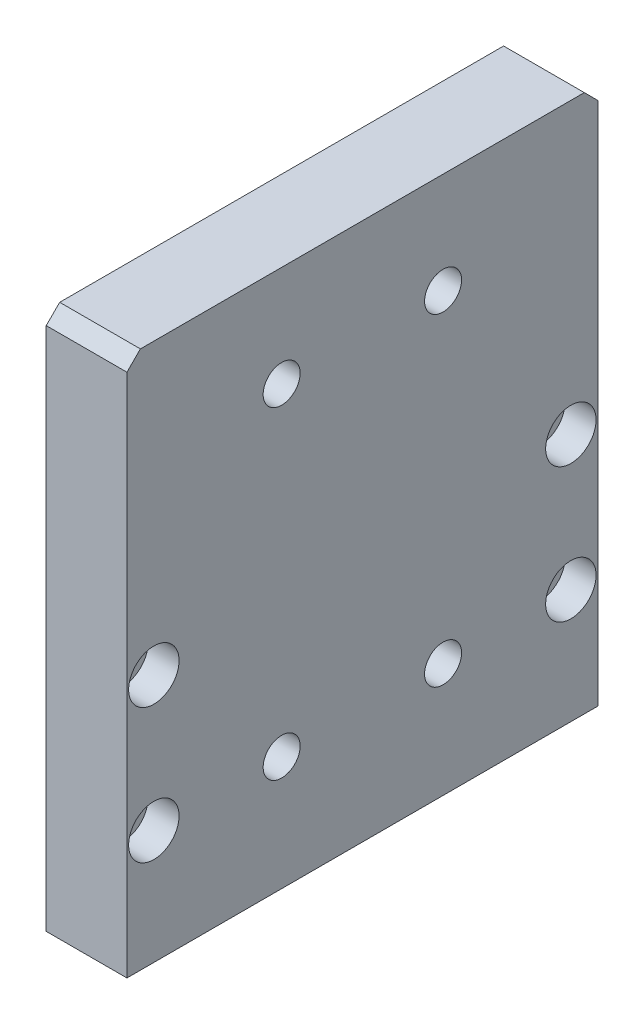
from build123d import *

# Parameters (mm, degrees)
SKETCH_1_W                   = 70
SKETCH_1_H                   = 80
EXTRUDE_1_DEPTH              = 12
HOLE_WIZARD_M5_1_D           = 5.5
HOLE_WIZARD_M5_1_CBORE_D     = 10
HOLE_WIZARD_M5_1_CBORE_DEPTH = 5.7
HOLE_WIZARD_M4_1_D           = 4.5
HOLE_WIZARD_M4_1_CBORE_D     = 7.5
HOLE_WIZARD_M4_1_CBORE_DEPTH = 4.6
HOLE_WIZARD_M4_1_2_D         = 3.3
HOLE_WIZARD_M4_1_2_DEPTH     = 10.1
HOLE_WIZARD_M4_1_2_TIP       = 0.991420021
CHAMFER_1_SIZE               = 2


with BuildPart() as part:
    # 草图1 → 凸台-拉伸1 (new body)
    with BuildSketch(Plane(origin=(0, 0, 0), x_dir=(0, 0, -1), z_dir=(1, 0, 0))):
        Rectangle(SKETCH_1_W, SKETCH_1_H)
    extrude(amount=EXTRUDE_1_DEPTH)

    # M5 六角圆柱头螺钉的柱形沉头孔1 (through all)
    with Locations(Plane.ZY):
        with Locations((-12, 25), (-12, -23), (12, -23), (12, 25)):
            CounterBoreHole(HOLE_WIZARD_M5_1_D / 2, HOLE_WIZARD_M5_1_CBORE_D / 2, HOLE_WIZARD_M5_1_CBORE_DEPTH)

    # Hole Wizard M4 _1 (through all)
    with Locations(Plane(origin=(12, 0, 0), x_dir=(0, 0, -1), z_dir=(1, 0, 0))):
        with Locations((-31, -23), (-31, -3), (31, -3), (31, -23)):
            CounterBoreHole(HOLE_WIZARD_M4_1_D / 2, HOLE_WIZARD_M4_1_CBORE_D / 2, HOLE_WIZARD_M4_1_CBORE_DEPTH)

    # Hole Wizard M4 _1 2
    with Locations(Plane(origin=(0, -40, 0), x_dir=(-1, 0, 0), z_dir=(0, -1, 0))):
        with Locations((-6, 22.5), (-6, -22.5)):
            Hole(HOLE_WIZARD_M4_1_2_D / 2, depth=HOLE_WIZARD_M4_1_2_DEPTH)
            with Locations((0, 0, -(HOLE_WIZARD_M4_1_2_DEPTH + HOLE_WIZARD_M4_1_2_TIP / 2))):  # 118° drill point
                Cone(0, HOLE_WIZARD_M4_1_2_D / 2, HOLE_WIZARD_M4_1_2_TIP, mode=Mode.SUBTRACT)

    # 倒角1
    chamfer_1_edges = [part.edges().sort_by_distance(p)[0] for p in [
        (6, 40, 35),
        (6, 40, -35),
    ]]
    chamfer(chamfer_1_edges, length=CHAMFER_1_SIZE)


solid = part.part
